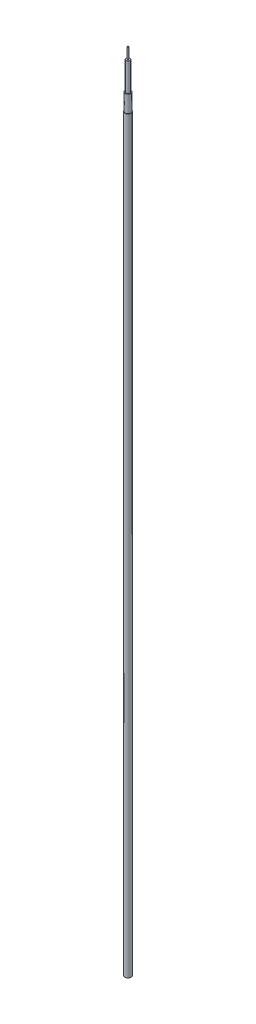
SolidWorks part; units mm, degrees
ref_plane "前视基准面" through (0, 0, 0) normal (0, 0, 1) x (1, 0, 0)
ref_plane "上视基准面" through (0, 0, 0) normal (0, 1, 0) x (1, 0, 0)
ref_plane "右视基准面" through (0, 0, 0) normal (1, 0, 0) x (0, 0, -1)
sketch "草图1" plane through (0, 0, 0) normal (0, 1, 0) x (1, 0, 0)
  circle A0 centre (0, 0) radius 0.565
  dimension "D1" = 1.13
extrude "凸台-拉伸1" add sketch "草图1" along normal blind 133
sketch "草图2" plane through (0, 133, 0) normal (0, 1, 0) x (1, 0, 0)
  circle A0 centre (0, 0) radius 0.5
extrude "凸台-拉伸2" add sketch "草图2" along normal blind 3
sketch "草图3" plane through (0, 136, 0) normal (0, 1, 0) x (1, 0, 0)
  circle A0 centre (0, 0) radius 0.35
  dimension "D1" = 0.7
extrude "凸台-拉伸3" add sketch "草图3" along normal blind 5
sketch "草图5" plane through (0, 141, 0) normal (0, 1, 0) x (1, 0, 0)
  circle A0 centre (0, 0) radius 0.1
  dimension "D1" = 0.2
extrude "凸台-拉伸4" add sketch "草图5" along normal blind 2
